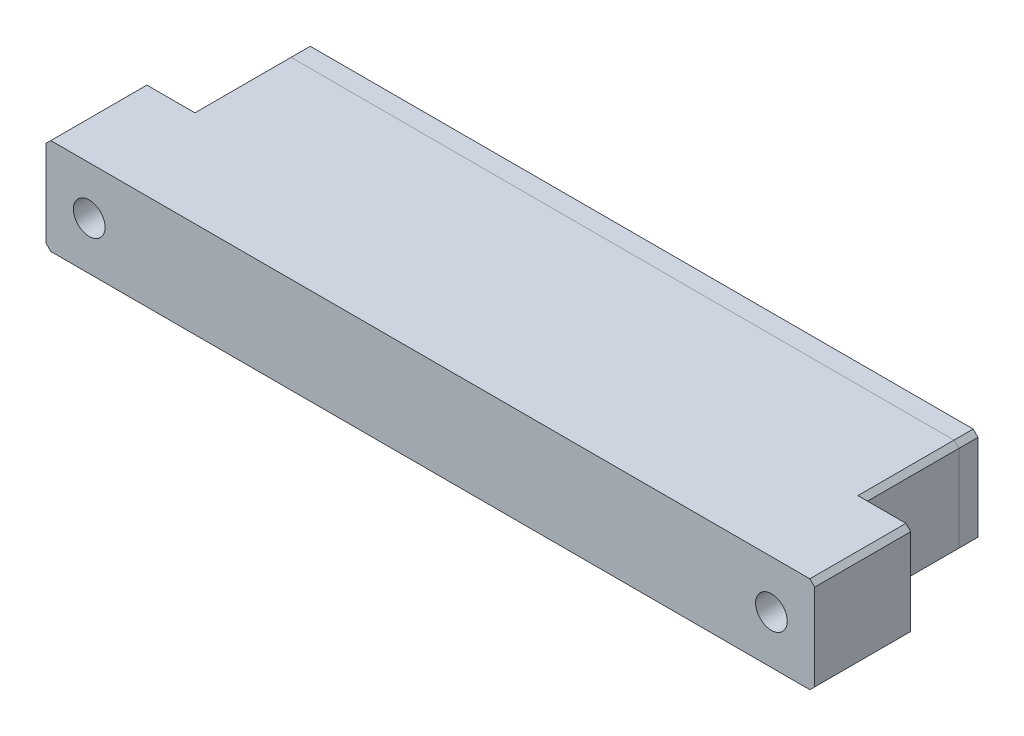
from build123d import *

# Parameters (mm, degrees)
SKETCH1_W             = 80
SKETCH1_H             = 10
BOSS_EXTRUDE1_DEPTH   = 20
SKETCH9_W             = 5
SKETCH9_H             = 10
CUT_EXTRUDE3_DEPTH    = 46.82575695
M4_TAPPED_HOLE1_D     = 3.3
M4_TAPPED_HOLE1_DEPTH = 8
M4_TAPPED_HOLE1_TIP   = 0.991420021
M5_TAPPED_HOLE1_D     = 4.2
M5_TAPPED_HOLE1_DEPTH = 8
SKETCH8_W             = 68
SKETCH8_H             = 8
CUT_EXTRUDE2_DEPTH    = 3
SKETCH10_W            = 64
SKETCH10_H            = 6
CUT_EXTRUDE4_DEPTH    = 3.5
SKETCH11_W            = 68
SKETCH11_H            = 8
BOSS_EXTRUDE2_DEPTH   = 3
SKETCH12_W            = 70
SKETCH12_H            = 10
BOSS_EXTRUDE3_DEPTH   = 2
SKETCH13_R            = 0.5
CUT_EXTRUDE5_DEPTH    = 5
LPATTERN1_COUNT       = 22
LPATTERN1_PITCH       = 3
CHAMFER1_SIZE         = 0.5
CHAMFER2_SIZE         = 0.5


with BuildPart() as part:
    # Sketch1 → Boss-Extrude1 (new body)
    with BuildSketch(Plane.XY):
        Rectangle(SKETCH1_W, SKETCH1_H)
    extrude(amount=BOSS_EXTRUDE1_DEPTH)

    # Sketch9 → Cut-Extrude3 (cut, through all)
    with BuildSketch(Plane(origin=(0, 5, 0), x_dir=(1, 0, 0), z_dir=(0, 1, 0))):
        with Locations((37.5, -5)):
            Rectangle(SKETCH9_W, SKETCH9_H)
        with Locations((-37.5, -5)):
            Rectangle(SKETCH9_W, SKETCH9_H)
    extrude(amount=-CUT_EXTRUDE3_DEPTH, mode=Mode.SUBTRACT)

    # M4 Tapped Hole1
    with Locations(Plane.XY.offset(20)):
        with Locations((-35.5, 0), (35.5, 0)):
            Hole(M4_TAPPED_HOLE1_D / 2, depth=M4_TAPPED_HOLE1_DEPTH)
            with Locations((0, 0, -(M4_TAPPED_HOLE1_DEPTH + M4_TAPPED_HOLE1_TIP / 2))):  # 118° drill point
                Cone(0, M4_TAPPED_HOLE1_D / 2, M4_TAPPED_HOLE1_TIP, mode=Mode.SUBTRACT)

    # M5 Tapped Hole1
    with Locations(Plane.XZ.offset(5)):
        with Locations((0, 6.5)):
            Hole(M5_TAPPED_HOLE1_D / 2, depth=M5_TAPPED_HOLE1_DEPTH)

    # Sketch8 → Cut-Extrude2 (cut)
    with BuildSketch(Plane(origin=(0, 0, 0), x_dir=(-1, 0, 0), z_dir=(0, 0, -1))):
        Rectangle(SKETCH8_W, SKETCH8_H)
    extrude(amount=-CUT_EXTRUDE2_DEPTH, mode=Mode.SUBTRACT)

    # Sketch10 → Cut-Extrude4 (cut)
    with BuildSketch(Plane(origin=(0, 0, 3), x_dir=(-1, 0, 0), z_dir=(0, 0, -1))):
        Rectangle(SKETCH10_W, SKETCH10_H)
    extrude(amount=-CUT_EXTRUDE4_DEPTH, mode=Mode.SUBTRACT)

    # Chamfer1
    chamfer1_edges = [part.edges().sort_by_distance(p)[0] for p in [
        (35, -5, 5),
        (35, 5, 5),
        (-35, -5, 5),
        (-35, 5, 5),
        (-40, 5, 15),
        (40, 5, 15),
        (40, -5, 15),
        (-40, -5, 15),
    ]]
    chamfer(chamfer1_edges, length=CHAMFER1_SIZE)


with BuildPart() as body_2:
    # Sketch11 → Boss-Extrude2 (new body)
    with BuildSketch(Plane(origin=(0, 0, 3), x_dir=(-1, 0, 0), z_dir=(0, 0, -1))):
        Rectangle(SKETCH11_W, SKETCH11_H)
    extrude(amount=BOSS_EXTRUDE2_DEPTH)


with BuildPart() as body_3:
    # Sketch12 → Boss-Extrude3 (new body)
    with BuildSketch(Plane(origin=(0, 0, 0), x_dir=(-1, 0, 0), z_dir=(0, 0, -1))):
        Rectangle(SKETCH12_W, SKETCH12_H)
    extrude(amount=BOSS_EXTRUDE3_DEPTH)


with BuildPart() as cut_extrude5_tool:
    # Sketch13 → Cut-Extrude5 (new body)
    with BuildSketch(Plane(origin=(0, 0, -2), x_dir=(-1, 0, 0), z_dir=(0, 0, -1))):
        with Locations((31.5, 1.5)):
            Circle(SKETCH13_R)
        with Locations((31.5, -1.5)):
            Circle(SKETCH13_R)
    cut_extrude5 = extrude(amount=-CUT_EXTRUDE5_DEPTH)


with BuildPart() as body_2_1:
    add(body_2.part)

    # Cut-Extrude5: cut by cut_extrude5_tool
    add(cut_extrude5_tool.part, mode=Mode.SUBTRACT)


with BuildPart() as body_3_1:
    add(body_3.part)

    # Cut-Extrude5: cut by cut_extrude5_tool
    add(cut_extrude5_tool.part, mode=Mode.SUBTRACT)


with BuildPart() as lpattern1_tool:
    # LPattern1: Cut-Extrude5 ×22
    with Locations(*[(i * LPATTERN1_PITCH, 0, 0) for i in range(1, LPATTERN1_COUNT)]):
        add(cut_extrude5)


with BuildPart() as body_2_2:
    add(body_2_1.part)

    # LPattern1: cut by lpattern1_tool
    add(lpattern1_tool.part, mode=Mode.SUBTRACT)


with BuildPart() as body_3_2:
    add(body_3_1.part)

    # LPattern1: cut by lpattern1_tool
    add(lpattern1_tool.part, mode=Mode.SUBTRACT)

    # Chamfer2
    chamfer2_edges = [body_3_2.edges().sort_by_distance(p)[0] for p in [
        (35, 5, -1),
        (-35, 5, -1),
        (-35, -5, -1),
        (35, -5, -1),
    ]]
    chamfer(chamfer2_edges, length=CHAMFER2_SIZE)


solid = Compound([part.part, body_2_2.part, body_3_2.part])
